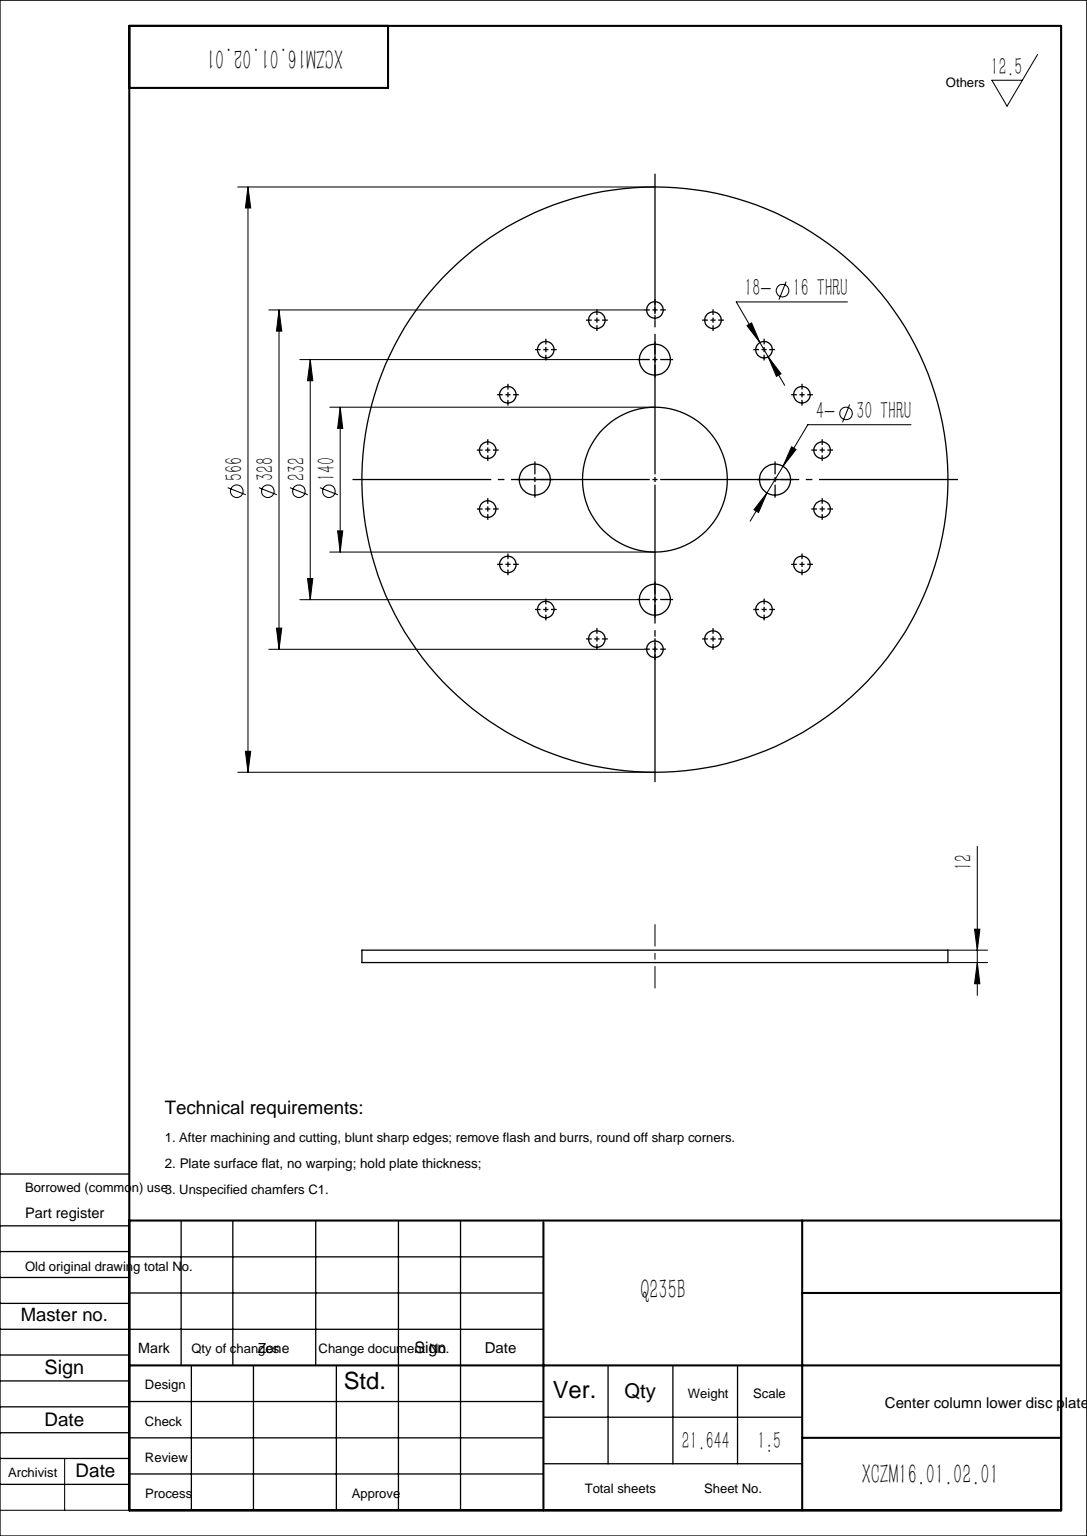
from build123d import *

# Parameters (mm, degrees)
SKETCH1_R           = 283
SKETCH1_R_2         = 70
SKETCH1_R_3         = 15
SKETCH1_R_4         = 8
BOSS_EXTRUDE1_DEPTH = 12


with BuildPart() as part:
    # Sketch1 → Boss-Extrude1 (new body)
    with BuildSketch(Plane(origin=(0, 0, 0), x_dir=(1, 0, 0), z_dir=(0, 1, 0))):
        with Locations(Location((0, 0, 0), (0, 0, 270))):
            Circle(SKETCH1_R)
        with Locations(Location((0, 0, 0), (0, 0, 270))):
            Circle(SKETCH1_R_2, mode=Mode.SUBTRACT)
        with Locations(Location((0, 116, 0), (0, 0, 270))):
            Circle(SKETCH1_R_3, mode=Mode.SUBTRACT)
        with Locations(Location((0, 164, 0), (0, 0, 270))):
            Circle(SKETCH1_R_4, mode=Mode.SUBTRACT)
        with Locations(Location((56.091303505, 154.109589809, 0), (0, 0, 270))):
            Circle(SKETCH1_R_4, mode=Mode.SUBTRACT)
        with Locations(Location((105.417167989, 125.631288672, 0), (0, 0, 270))):
            Circle(SKETCH1_R_4, mode=Mode.SUBTRACT)
        with Locations(Location((142.028166221, 82, 0), (0, 0, 270))):
            Circle(SKETCH1_R_4, mode=Mode.SUBTRACT)
        with Locations(Location((161.508471494, 28.478301137, 0), (0, 0, 270))):
            Circle(SKETCH1_R_4, mode=Mode.SUBTRACT)
        with Locations(Location((161.508471494, -28.478301137, 0), (0, 0, 270))):
            Circle(SKETCH1_R_4, mode=Mode.SUBTRACT)
        with Locations(Location((142.028166221, -82, 0), (0, 0, 270))):
            Circle(SKETCH1_R_4, mode=Mode.SUBTRACT)
        with Locations(Location((105.417167989, -125.631288672, 0), (0, 0, 270))):
            Circle(SKETCH1_R_4, mode=Mode.SUBTRACT)
        with Locations(Location((56.091303505, -154.109589809, 0), (0, 0, 270))):
            Circle(SKETCH1_R_4, mode=Mode.SUBTRACT)
        with Locations(Location((0, -164, 0), (0, 0, 270))):
            Circle(SKETCH1_R_4, mode=Mode.SUBTRACT)
        with Locations(Location((-56.091303505, -154.109589809, 0), (0, 0, 270))):
            Circle(SKETCH1_R_4, mode=Mode.SUBTRACT)
        with Locations(Location((-105.417167989, -125.631288672, 0), (0, 0, 270))):
            Circle(SKETCH1_R_4, mode=Mode.SUBTRACT)
        with Locations(Location((-142.028166221, -82, 0), (0, 0, 270))):
            Circle(SKETCH1_R_4, mode=Mode.SUBTRACT)
        with Locations(Location((-161.508471494, -28.478301137, 0), (0, 0, 270))):
            Circle(SKETCH1_R_4, mode=Mode.SUBTRACT)
        with Locations(Location((-161.508471494, 28.478301137, 0), (0, 0, 270))):
            Circle(SKETCH1_R_4, mode=Mode.SUBTRACT)
        with Locations(Location((-142.028166221, 82, 0), (0, 0, 270))):
            Circle(SKETCH1_R_4, mode=Mode.SUBTRACT)
        with Locations(Location((-105.417167989, 125.631288672, 0), (0, 0, 270))):
            Circle(SKETCH1_R_4, mode=Mode.SUBTRACT)
        with Locations(Location((-56.091303505, 154.109589809, 0), (0, 0, 270))):
            Circle(SKETCH1_R_4, mode=Mode.SUBTRACT)
        with Locations(Location((116, 0, 0), (0, 0, 270))):
            Circle(SKETCH1_R_3, mode=Mode.SUBTRACT)
        with Locations(Location((0, -116, 0), (0, 0, 270))):
            Circle(SKETCH1_R_3, mode=Mode.SUBTRACT)
        with Locations(Location((-116, 0, 0), (0, 0, 270))):
            Circle(SKETCH1_R_3, mode=Mode.SUBTRACT)
    extrude(amount=BOSS_EXTRUDE1_DEPTH)


solid = part.part
